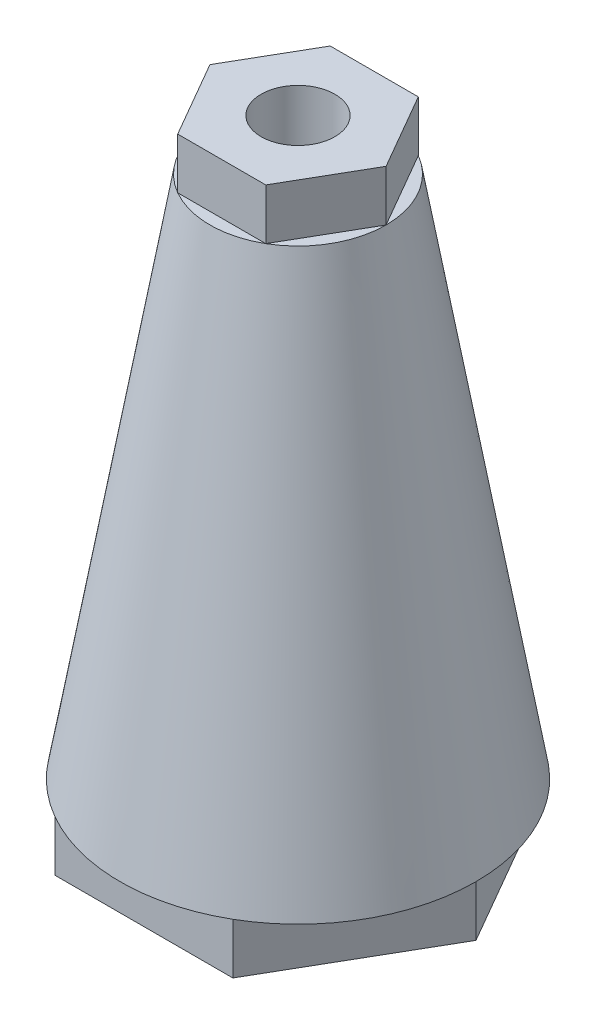
from build123d import *

# Parameters (mm, degrees)
BOSS_EXTRUDE1_DEPTH    = 10
BOSS_EXTRUDE2_DEPTH    = 10
M16X1_5_TAPPED_HOLE1_D = 14.5


with BuildPart() as part:
    # Sketch1 → Boss-Extrude1 (new body)
    with BuildSketch(Plane(origin=(0, 0, 0), x_dir=(1, 0, 0), z_dir=(0, 1, 0))):
        Polygon((8.660254038, -15), (17.320508076, 0), (8.660254038, 15), (-8.660254038, 15), (-17.320508076, 0), (-8.660254038, -15), align=None)
    extrude(amount=BOSS_EXTRUDE1_DEPTH)

    # Sketch4 → Revolve1 (revolve)
    with BuildSketch(Plane.XY, mode=Mode.PRIVATE) as revolve1_sk:
        Polygon((0, 0), (17.320508076, 0), (35, -103), (0, -103), align=None)
    revolve(revolve1_sk.sketch.rotate(Axis((0, -103, 0), (0, 1, 0)), 90), axis=Axis((0, -103, 0), (0, 1, 0)))

    # Sketch7 → Boss-Extrude2 (add)
    with BuildSketch(Plane.XZ.offset(103)):
        Polygon((17.5, 30.310889132), (-17.5, 30.310889132), (-35, 0), (-17.5, -30.310889132), (17.5, -30.310889132), (35, 0), align=None)
    extrude(amount=BOSS_EXTRUDE2_DEPTH)

    # M16x1.5 Tapped Hole1 (through all)
    with Locations(Plane(origin=(0, 10, 0), x_dir=(1, 0, 0), z_dir=(0, 1, 0))):
        with Locations((0, 0)):
            Hole(M16X1_5_TAPPED_HOLE1_D / 2)


solid = part.part
